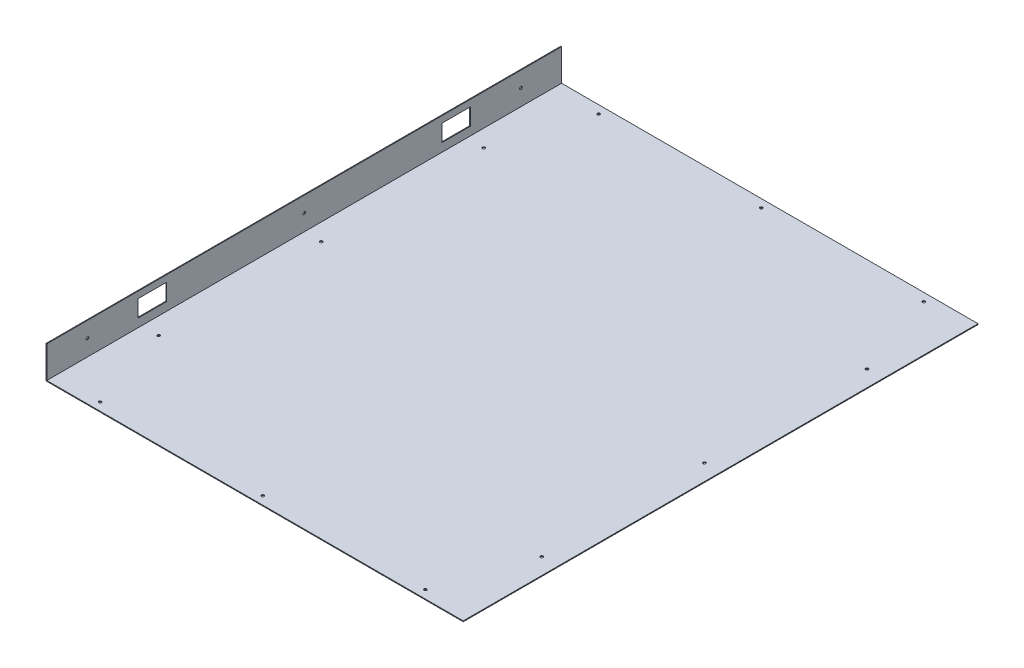
from build123d import *

# Parameters (mm, degrees)
BOSS_EXTRUDE1_DEPTH = 950
SKETCH2_R           = 2.5
SKETCH2_W           = 53
SKETCH2_H           = 31
CUT_EXTRUDE1_DEPTH  = 1356.5
SKETCH3_R           = 2.5
CUT_EXTRUDE2_DEPTH  = 1.5
SKETCH5_W           = 1.5
SKETCH5_H           = 950
CUT_EXTRUDE4_DEPTH  = 58.5


with BuildPart() as part:
    # Sketch1 → Boss-Extrude1 (new body)
    with BuildSketch(Plane.XY):
        Polygon((0, 0), (0, -60), (770, -60), (770, 0), (768.5, 0), (768.5, -58.5), (1.5, -58.5), (1.5, 0), align=None)
    extrude(amount=BOSS_EXTRUDE1_DEPTH)

    # Sketch2 → Cut-Extrude1 (cut)
    with BuildSketch(Plane(origin=(770, 0, 0), x_dir=(0, 0, -1), z_dir=(1, 0, 0))):
        with Locations(Location((-75, -28.5, 0), (0, 0, 270))):
            Circle(SKETCH2_R)
        with Locations(Location((-475, -28.5, 0), (0, 0, 270))):
            Circle(SKETCH2_R)
        with Locations(Location((-875, -28.5, 0), (0, 0, 270))):
            Circle(SKETCH2_R)
        with Locations((-194.5, -27.5)):
            Rectangle(SKETCH2_W, SKETCH2_H)
        with Locations((-755.5, -27.5)):
            Rectangle(SKETCH2_W, SKETCH2_H)
    extrude(amount=-CUT_EXTRUDE1_DEPTH, mode=Mode.SUBTRACT)

    # Sketch3 → Cut-Extrude2 (cut)
    with BuildSketch(Plane.XZ.offset(60)):
        with Locations(Location((740, 475, 0), (0, 0, 270))):
            Circle(SKETCH3_R)
        with Locations(Location((740, 775, 0), (0, 0, 270))):
            Circle(SKETCH3_R)
        with Locations(Location((740, 175, 0), (0, 0, 270))):
            Circle(SKETCH3_R)
        with Locations(Location((33, 775, 0), (0, 0, 270))):
            Circle(SKETCH3_R)
        with Locations(Location((33, 475, 0), (0, 0, 270))):
            Circle(SKETCH3_R)
        with Locations(Location((33, 175, 0), (0, 0, 270))):
            Circle(SKETCH3_R)
        with Locations(Location((385, 935, 0), (0, 0, 270))):
            Circle(SKETCH3_R)
        with Locations(Location((685, 935, 0), (0, 0, 270))):
            Circle(SKETCH3_R)
        with Locations(Location((85, 935, 0), (0, 0, 270))):
            Circle(SKETCH3_R)
        with Locations(Location((85, 15, 0), (0, 0, 90))):
            Circle(SKETCH3_R)
        with Locations(Location((685, 15, 0), (0, 0, 90))):
            Circle(SKETCH3_R)
        with Locations(Location((385, 15, 0), (0, 0, 90))):
            Circle(SKETCH3_R)
    extrude(amount=-CUT_EXTRUDE2_DEPTH, mode=Mode.SUBTRACT)

    # Sketch5 → Cut-Extrude4 (cut)
    with BuildSketch(Plane(origin=(0, 0, 0), x_dir=(1, 0, 0), z_dir=(0, 1, 0))):
        with Locations((769.25, -475)):
            Rectangle(SKETCH5_W, SKETCH5_H)
    extrude(amount=-CUT_EXTRUDE4_DEPTH, mode=Mode.SUBTRACT)


solid = part.part
